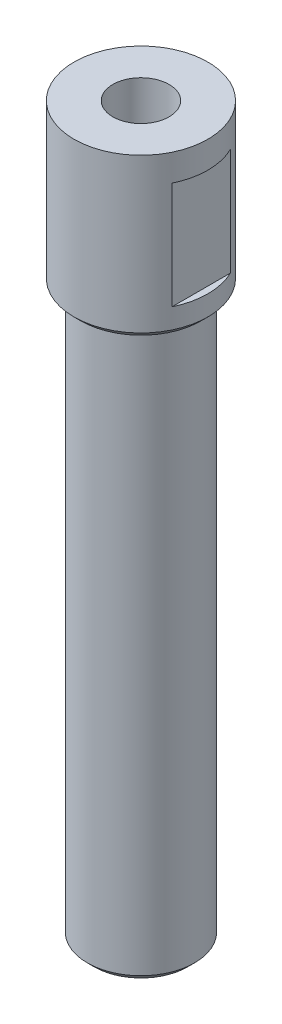
SolidWorks part; units mm, degrees
ref_plane "Front Plane" through (0, 0, 0) normal (0, 0, 1) x (1, 0, 0)
ref_plane "Top Plane" through (0, 0, 0) normal (0, 1, 0) x (1, 0, 0)
ref_plane "Right Plane" through (0, 0, 0) normal (1, 0, 0) x (0, 0, -1)
sketch "Sketch1" plane through (0, 0, 0) normal (0, 1, 0) x (1, 0, 0)
  circle A0 centre (0, 0) radius 4
  dimension "D1" = 8
extrude "Boss-Extrude1" add sketch "Sketch1" along normal blind 42.3
sketch "Sketch2" plane through (0, 42.3, 0) normal (0, 1, 0) x (1, 0, 0)
  circle A0 centre (0, 0) radius 5
  dimension "D1" = 10
extrude "Boss-Extrude2" add sketch "Sketch2" along normal blind 12
hole_wizard "M5 Tapped Hole1" positions "3DSketch1" profile "Sketch3" tap size "M5" standard "Gb"
sketch3d "3DSketch1"
  line L0 (0, 54.3, 0) -> (0, 42.3, 0) construction
  point P0 (0, 54.3, 0)
sketch "Sketch3" plane through (0, 54.3, 0) normal (1, 0, 0) x (0, 0, 1)
  line L0 (0, 0) -> (0, 13.6618)
  line L1 (0, 13.6618) -> (2.1, 12.4)
  line L2 (2.1, 12.4) -> (2.1, 0)
  line L5 (2.1, 0) -> (0, 0)
  line L10 (0, 13.6618) -> (-2.1, 12.4) construction
  line L11 (0, -6.35) -> (0, 107.95) construction
  dimension "螺纹孔钻头直径" = 4.2
  dimension "螺纹孔钻头深度" = 12.4
  dimension "导头角度" = 118
cosmetic thread "Cosmetic thread 1" parameters "D1"=10, "D2"=5
hole_wizard "M4 Tapped Hole1" positions "3DSketch2" profile "Sketch4" tap size "M4" standard "Gb"
sketch3d "3DSketch2"
  point P0 (0, 0, 0)
  point P3 (0, 0, 0)
  dimension "D1" = 0
sketch "Sketch4" plane through (0, 0, 0) normal (1, 0, 0) x (0, 0, -1)
  line L0 (0, 0) -> (0, 11.0914)
  line L1 (0, 11.0914) -> (1.65, 10.1)
  line L2 (1.65, 10.1) -> (1.65, 0)
  line L5 (1.65, 0) -> (0, 0)
  line L10 (0, 11.0914) -> (-1.65, 10.1) construction
  line L11 (0, -6.35) -> (0, 107.95) construction
  dimension "螺纹孔钻头直径" = 3.3
  dimension "螺纹孔钻头深度" = 10.1
  dimension "导头角度" = 118
cosmetic thread "Cosmetic thread 2" parameters "D1"=8, "D2"=4
cosmetic thread "Cosmetic thread 3" parameters "D1"=8, "D2"=4
sketch "Sketch5" plane through (0, 0, 0) normal (0, 0, 1) x (1, 0, 0)
  line L0 (0, 54.3) -> (0, -49945.7) construction
  line L1 (2.1, 54.3) -> (-2.1, 54.3) construction
  line L2 (-5, 54.3) -> (-5, 42.3) construction
  line L3 (-5.5, 52.3) -> (-4.5, 52.3)
  line L4 (-5.5, 52.3) -> (-5.5, 44.3)
  line L5 (-5.5, 44.3) -> (-4.5, 44.3)
  line L6 (-4.5, 52.3) -> (-4.5, 44.3)
  line L7 (-5.5, 52.3) -> (-4.5, 44.3) construction
  line L8 (-5.5, 44.3) -> (-4.5, 52.3) construction
  line L9 (5.5, 44.3) -> (4.5, 52.3) construction
  line L10 (5.5, 52.3) -> (4.5, 44.3) construction
  line L11 (4.5, 52.3) -> (4.5, 44.3)
  line L12 (5.5, 44.3) -> (4.5, 44.3)
  line L13 (5.5, 52.3) -> (5.5, 44.3)
  line L14 (5.5, 52.3) -> (4.5, 52.3)
  point P4 (0, 54.3)
  point P5 (-5, 48.3)
  point P16 (5, 48.3)
  dimension "D1" = 8
  dimension "D2" = 9
extrude "Cut-Extrude1" cut sketch "Sketch5" against normal mid plane 10
chamfer "Chamfer1" distance 0.5 angle 45 2 edges at (0, 42.3, 5) (0, 0, 4)
